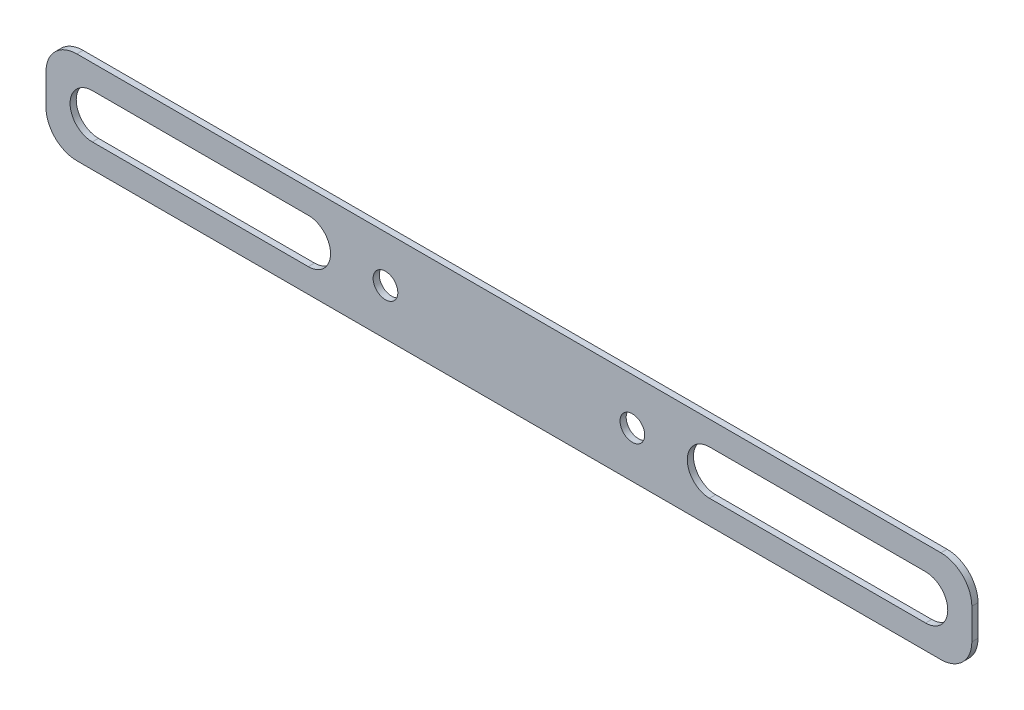
from build123d import *

# Parameters (mm, degrees)
SKETCH1_W           = 300
SKETCH1_H           = 30
BOSS_EXTRUDE1_DEPTH = 2
CUT_EXTRUDE1_DEPTH  = 151.761400896
FILLET1_R           = 10
FILLET2_R           = 10
SKETCH4_R           = 4
CUT_EXTRUDE2_DEPTH  = 151.761400896


with BuildPart() as part:
    # Sketch1 → Boss-Extrude1 (new body)
    with BuildSketch(Plane.XY):
        Rectangle(SKETCH1_W, SKETCH1_H)
    extrude(amount=BOSS_EXTRUDE1_DEPTH)

    # Sketch2 → Cut-Extrude1 (cut, through all)
    with BuildSketch(Plane.XY.offset(2)):
        with BuildLine():
            Line((-135, 7.2), (-65, 7.2))
            ThreePointArc((-65, 7.2), (-57.8, 0), (-65, -7.2))
            Line((-65, -7.2), (-135, -7.2))
            ThreePointArc((-135, -7.2), (-142.2, 0), (-135, 7.2))
        make_face()
    cut_extrude1 = extrude(amount=-CUT_EXTRUDE1_DEPTH, mode=Mode.SUBTRACT)

    # Fillet1
    fillet1_edges = [part.edges().sort_by_distance(p)[0] for p in [
        (-150, 15, 1),
        (-150, -15, 1),
    ]]
    fillet(fillet1_edges, radius=FILLET1_R)

    # Mirror1: Cut-Extrude1 across plane
    add(cut_extrude1.mirror(Plane(origin=(0, 0, 0), x_dir=(0, 0, 1), z_dir=(1, 0, 0))), mode=Mode.SUBTRACT)

    # Fillet2
    fillet2_edges = [part.edges().sort_by_distance(p)[0] for p in [
        (150, 15, 1),
        (150, -15, 1),
    ]]
    fillet(fillet2_edges, radius=FILLET2_R)

    # Sketch4 → Cut-Extrude2 (cut, through all)
    with BuildSketch(Plane(origin=(0, 0, 0), x_dir=(-1, 0, 0), z_dir=(0, 0, -1))):
        with Locations((40, 0)):
            Circle(SKETCH4_R)
        with Locations((-40, 0)):
            Circle(SKETCH4_R)
    extrude(amount=-CUT_EXTRUDE2_DEPTH, mode=Mode.SUBTRACT)


solid = part.part
